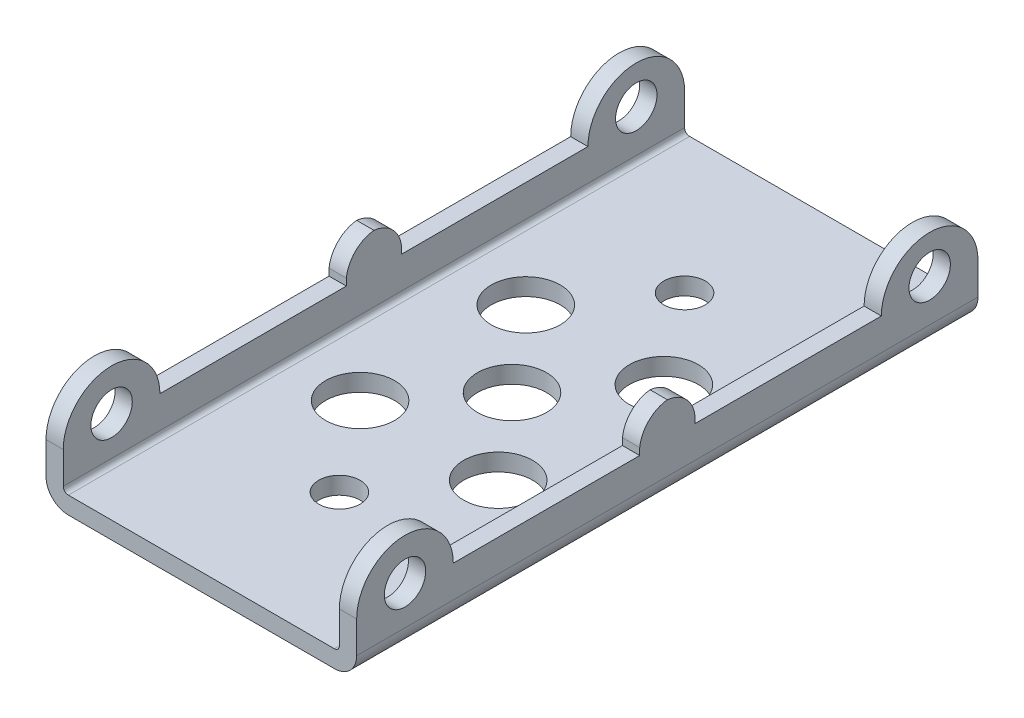
from build123d import *

# Parameters (mm, degrees)
BOSS_EXTRUDE1_DEPTH          = 2.5
SKETCH2_W                    = 90
SKETCH2_H                    = 2.5
BOSS_EXTRUDE2_DEPTH          = 40.000031182
BOSS_EXTRUDE3_DEPTH          = 2.5
F_6_0_6_DIAMETER_HOLE1_D     = 6
F_6_0_6_DIAMETER_HOLE1_DEPTH = 2.5
F_6_0_6_DIAMETER_HOLE2_D     = 6
F_6_0_6_DIAMETER_HOLE2_DEPTH = 2.5
F_10_0_10_DIAMETER_HOLE1_D   = 10
F_6_0_6_DIAMETER_HOLE3_D     = 6
FILLET1_R                    = 0.7366
FILLET2_R                    = 3.2366


with BuildPart() as part:
    # Sketch1 → Boss-Extrude1 (new body)
    with BuildSketch(Plane(origin=(-22.498134156, 0, 0), x_dir=(0, -1, 0), z_dir=(-1, 0, 0))):
        with BuildLine():
            Line((-5.354521861, -90), (2.5, -90))
            Line((2.5, -90), (2.5, 0))
            Line((2.5, 0), (-5.354521861, 0))
            ThreePointArc((-5.354521861, 0), (-12.354521861, -7), (-5.354521861, -14))
            Line((-5.354521861, -14), (-5.354521861, -41))
            Line((-5.354521861, -41), (-6.354521861, -41))
            ThreePointArc((-6.354521861, -41), (-9.05608398, -42.298437881), (-10.354521861, -45))
            ThreePointArc((-10.354521861, -45), (-9.05608398, -47.701562119), (-6.354521861, -49))
            Line((-6.354521861, -49), (-5.354521861, -49))
            Line((-5.354521861, -49), (-5.354521861, -76))
            ThreePointArc((-5.354521861, -76), (-12.354521861, -83), (-5.354521861, -90))
        make_face()
    extrude(amount=-BOSS_EXTRUDE1_DEPTH)

    # Sketch2 → Boss-Extrude2 (add)
    with BuildSketch(Plane(origin=(-19.998134156, 0, 0), x_dir=(0, 0, -1), z_dir=(1, 0, 0))):
        with Locations((45, -1.25)):
            Rectangle(SKETCH2_W, SKETCH2_H)
    extrude(amount=BOSS_EXTRUDE2_DEPTH)

    # Sketch3 → Boss-Extrude3 (add)
    with BuildSketch(Plane(origin=(20.001897026, 0, 0), x_dir=(0, 0, -1), z_dir=(1, 0, 0))):
        with BuildLine():
            Line((0, -2.5), (0, 5.350758991))
            ThreePointArc((0, 5.350758991), (7, 12.350758991), (14, 5.350758991))
            Line((14, 5.350758991), (41, 5.350758991))
            Line((41, 5.350758991), (41, 6.350758991))
            ThreePointArc((41, 6.350758991), (42.298437881, 9.05232111), (45, 10.350758991))
            ThreePointArc((45, 10.350758991), (47.701562119, 9.05232111), (49, 6.350758991))
            Line((49, 6.350758991), (49, 5.350758991))
            Line((49, 5.350758991), (76, 5.350758991))
            ThreePointArc((76, 5.350758991), (83, 12.350758991), (90, 5.350758991))
            Line((90, 5.350758991), (90, -2.5))
            Line((90, -2.5), (0, -2.5))
        make_face()
    extrude(amount=BOSS_EXTRUDE3_DEPTH)

    # Ø6.0 (6) Diameter Hole1
    with Locations(Plane.ZY.offset(-20.001897026)):
        with Locations((-83, 6.850758991), (-7, 6.350758991)):
            Hole(F_6_0_6_DIAMETER_HOLE1_D / 2, depth=F_6_0_6_DIAMETER_HOLE1_DEPTH)

    # Ø6.0 (6) Diameter Hole2
    with Locations(Plane(origin=(-19.998134156, 0, 0), x_dir=(0, 0, -1), z_dir=(1, 0, 0))):
        with Locations((83, 6.854521861), (7, 6.354521861)):
            Hole(F_6_0_6_DIAMETER_HOLE2_D / 2, depth=F_6_0_6_DIAMETER_HOLE2_DEPTH)

    # Ø10.0 (10) Diameter Hole1 (through all)
    with Locations(Plane(origin=(0, 0, 0), x_dir=(1, 0, 0), z_dir=(0, 1, 0))):
        with Locations((0, 45), (-10, 57), (-10, 33), (10, 33), (10, 57)):
            Hole(F_10_0_10_DIAMETER_HOLE1_D / 2)

    # Ø6.0 (6) Diameter Hole3 (through all)
    with Locations(Plane(origin=(0, 0, 0), x_dir=(1, 0, 0), z_dir=(0, 1, 0))):
        with Locations((0, 70), (0, 20)):
            Hole(F_6_0_6_DIAMETER_HOLE3_D / 2)

    # Fillet1
    fillet1_edges = [part.edges().sort_by_distance(p)[0] for p in [
        (-19.998134156, 0, -45),
        (20.001897026, 0, -45),
    ]]
    fillet(fillet1_edges, radius=FILLET1_R)

    # Fillet2
    fillet2_edges = [part.edges().sort_by_distance(p)[0] for p in [
        (-22.498134156, -2.5, -45),
        (22.501897026, -2.5, -45),
    ]]
    fillet(fillet2_edges, radius=FILLET2_R)


solid = part.part
